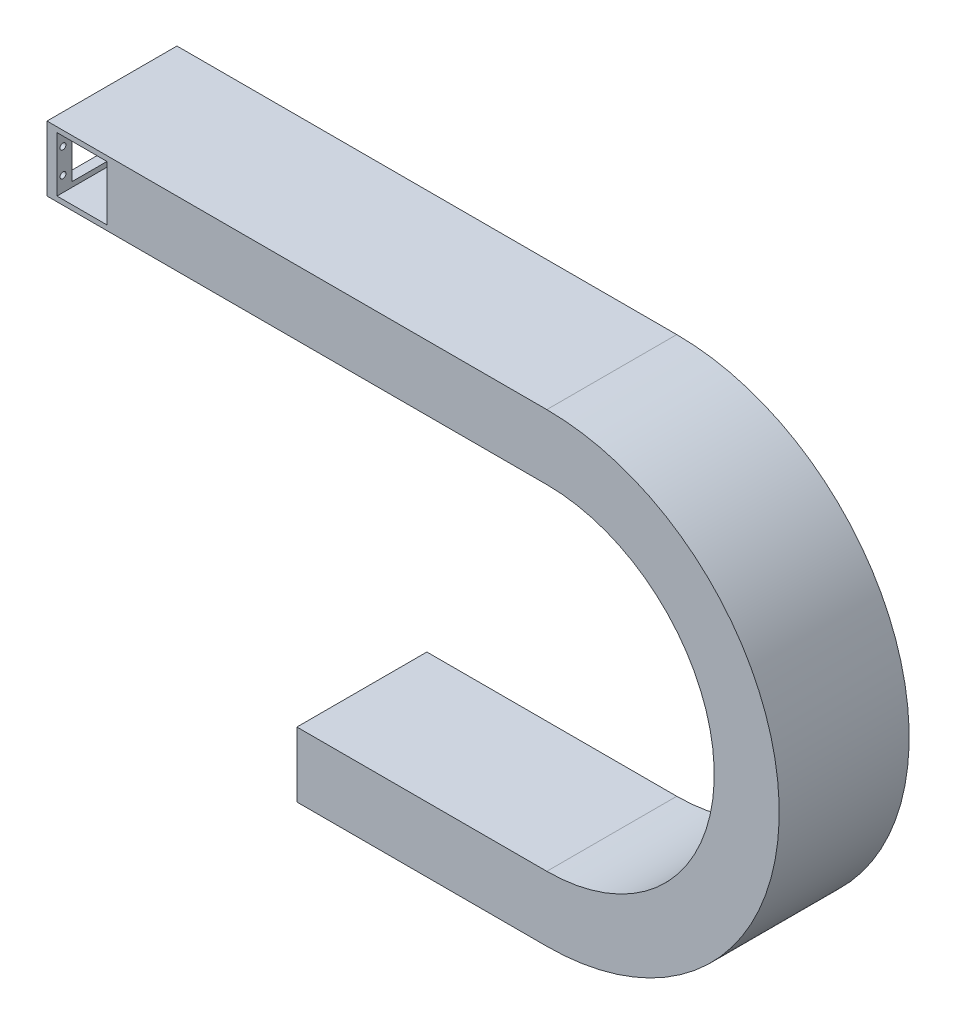
SolidWorks part; units mm, degrees
ref_plane "前视基准面" through (0, 0, 0) normal (0, 0, 1) x (1, 0, 0)
ref_plane "上视基准面" through (0, 0, 0) normal (0, 1, 0) x (1, 0, 0)
ref_plane "右视基准面" through (0, 0, 0) normal (1, 0, 0) x (0, 0, -1)
sketch "草图1" plane through (0, 0, 0) normal (0, 0, 1) x (1, 0, 0)
  line L0 (-450.4277, 234.0221) -> (-950.4277, 234.0221)
  line L1 (-450.4277, -100.9779) -> (-700.4277, -100.9779)
  line L2 (-450.4277, -165.9779) -> (-700.4277, -165.9779)
  line L3 (-450.4277, 299.0221) -> (-950.4277, 299.0221)
  line L4 (-950.4277, 299.0221) -> (-950.4277, 234.0221)
  line L5 (-700.4277, -165.9779) -> (-700.4277, -100.9779)
  arc A0 (-450.4277, -100.9779) -> (-450.4277, 234.0221) centre (-450.4277, 66.5221) ccw
  arc A1 (-450.4277, -165.9779) -> (-450.4277, 299.0221) centre (-450.4277, 66.5221) ccw
  dimension "D1" = 500
  dimension "D4" = 167.5
  dimension "D2" = 250
  dimension "D3" = 65
extrude "凸台-拉伸1" add sketch "草图1" along normal blind 130
sketch "草图2" plane through (-950.4277, 0, 0) normal (-1, 0, 0) x (0, 0, 1)
  line L0 (130, 299.0221) -> (0, 299.0221) construction
  line L1 (130, 299.0221) -> (130, 234.0221) construction
  circle A0 centre (6, 279.0221) radius 3
  circle A1 centre (6, 254.0221) radius 3
  circle A2 centre (124, 279.0221) radius 3
  circle A3 centre (124, 254.0221) radius 3
  dimension "D1" = 25
  dimension "D2" = 25
  dimension "D3" = 6
  dimension "D4" = 118
  dimension "D5" = 20
  dimension "D6" = 6
  dimension "D8" = 118
  dimension "D7" = 20
extrude "切除-拉伸1" cut sketch "草图2" against normal blind 20
sketch "草图9" plane through (0, 0, 130) normal (0, 0, 1) x (1, 0, 0)
  line L0 (-450.4277, 299.0221) -> (-950.4277, 299.0221) construction
  line L1 (-940.4277, 294.0221) -> (-890.4277, 294.0221)
  line L2 (-940.4277, 294.0221) -> (-940.4277, 239.0221)
  line L3 (-940.4277, 239.0221) -> (-890.4277, 239.0221)
  line L4 (-890.4277, 294.0221) -> (-890.4277, 239.0221)
  line L5 (-950.4277, 234.0221) -> (-450.4277, 234.0221) construction
  line L6 (-950.4277, 299.0221) -> (-950.4277, 234.0221) construction
  dimension "D1" = 5
  dimension "D2" = 5
  dimension "D3" = 10
  dimension "D4" = 50
extrude "切除-拉伸2" cut sketch "草图9" against normal blind 150
sketch "草图10" plane through (-950.4277, 0, 0) normal (-1, 0, 0) x (0, 0, 1)
  line L0 (130, 299.0221) -> (0, 299.0221) construction
  line L1 (15, 289.0221) -> (115, 289.0221)
  line L2 (15, 289.0221) -> (15, 244.0221)
  line L3 (15, 244.0221) -> (115, 244.0221)
  line L4 (115, 289.0221) -> (115, 244.0221)
  line L5 (0, 299.0221) -> (0, 234.0221) construction
  dimension "D1" = 100
  dimension "D2" = 45
  dimension "D3" = 10
  dimension "D4" = 15
extrude "切除-拉伸3" cut sketch "草图10" against normal blind 200
